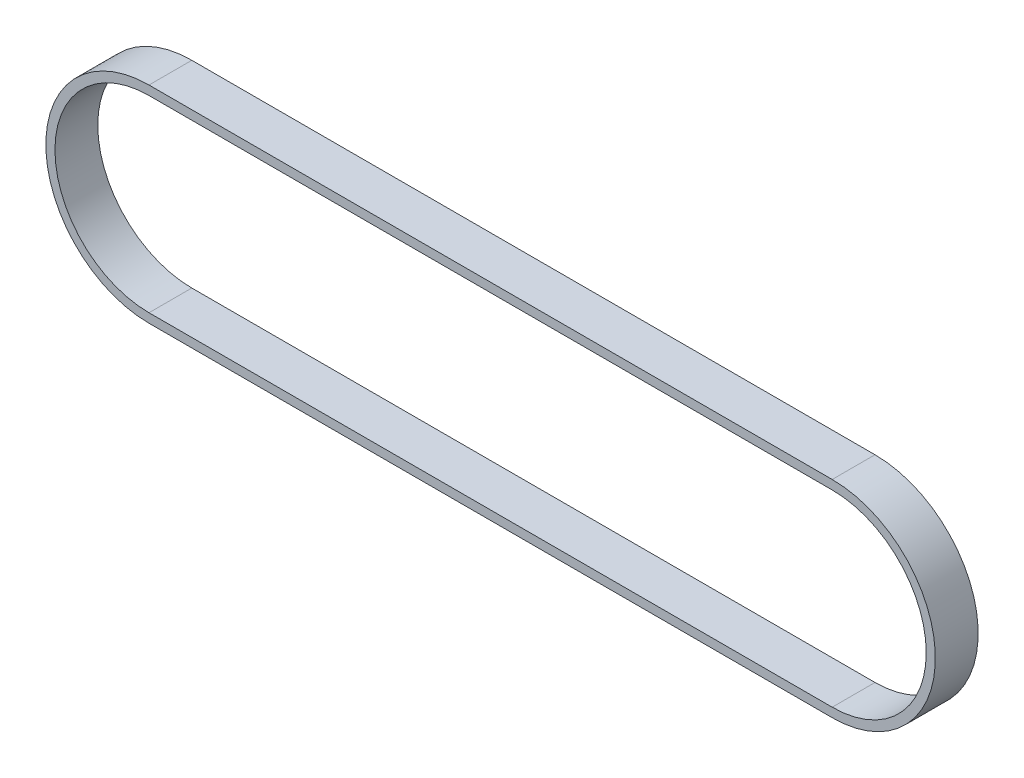
SolidWorks part; units mm, degrees
ref_plane "前视基准面" through (0, 0, 0) normal (0, 0, 1) x (1, 0, 0)
ref_plane "上视基准面" through (0, 0, 0) normal (0, 1, 0) x (1, 0, 0)
ref_plane "右视基准面" through (0, 0, 0) normal (1, 0, 0) x (0, 0, -1)
sketch "草图1" plane through (0, 0, 0) normal (0, 0, 1) x (1, 0, 0)
  line L0 (0, 0) -> (150, 0) construction
  line L1 (0, 21.65) -> (150, 21.65)
  line L2 (0, -21.65) -> (150, -21.65)
  arc A0 (0, 21.65) -> (0, -21.65) centre (0, 0) ccw
  arc A1 (150, -21.65) -> (150, 21.65) centre (150, 0) ccw
  point P3 (75, 0)
  dimension "D2" = 21.65
  dimension "D1" = 150
extrude "拉伸-薄壁1" add sketch "草图1" along normal mid plane 9.4 thin thin type mid plane wall 2
